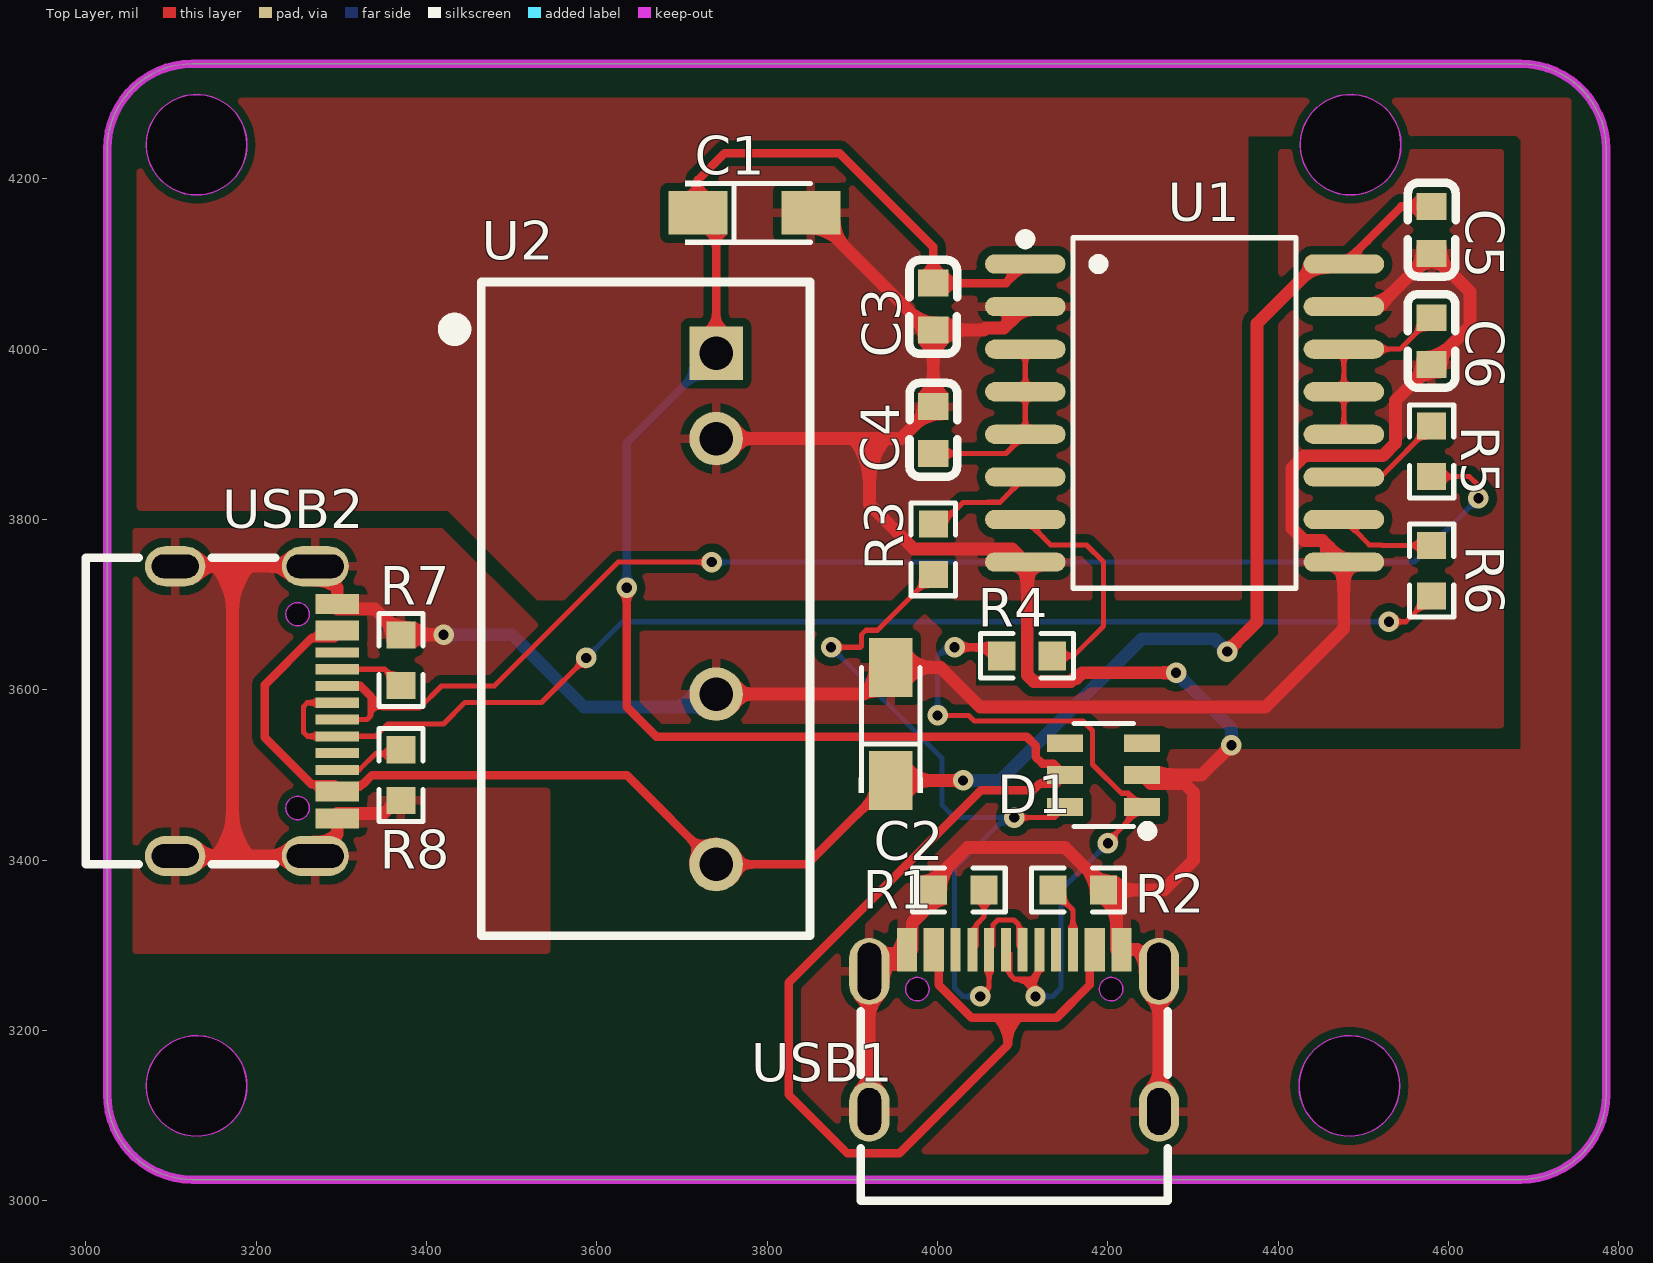
[diagram p0: Top Layer view]
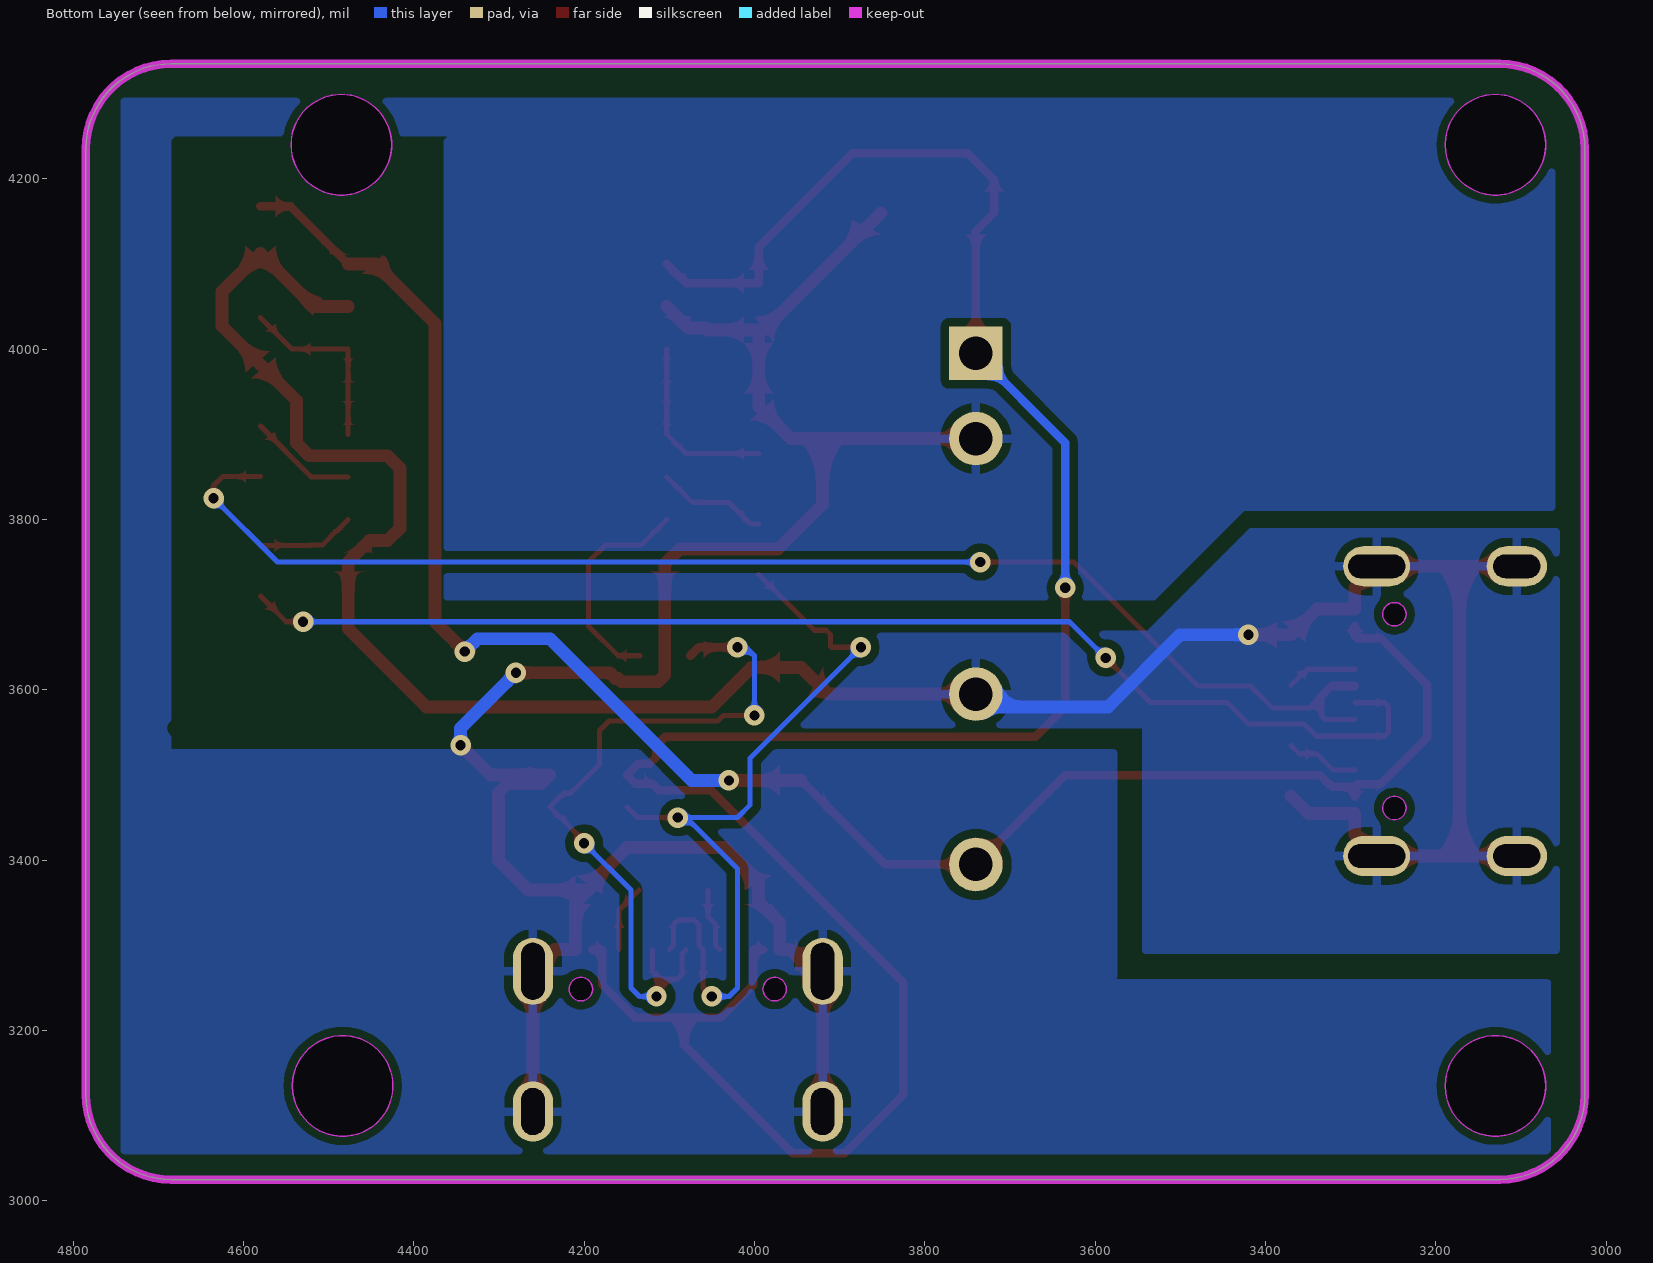
[diagram p1: Bottom Layer view, seen from below]
# Altium PCB MISC79005.pcbdoc
Units mil, origin at the board's own origin, x right, y up, seen from the top; angles counter-clockwise.
Board outline 1760 x 1310 mil, 2 copper layers (Top Layer, Bottom Layer), stack 62.206 mil thick; 19 components, 18 nets, 94 pads, 17 vias.

## Layer stack, top to bottom
Top Solder Mask Layer: solder mask 0.394, Dk 3.3
Top Layer: signal copper 1.379
Dielectric1: surface 59.449, FR4, Dk 4.5
Bottom Layer: signal copper 1.378
Bottom Solder Mask Layer: solder mask 0.394, Dk 3.3

## Board outline
3125,4335 ccw(c3125,4235) 3025,4235 3025,3125 ccw(c3125,3125) 3125,3025 4685,3025 ccw(c4685,3125) 4785,3125 4785,4235 ccw(c4685,4235) 4685,4335
cut-out: 3189.1,4240 cw(c3130,4240) 3070.9,4240 cw(c3130,4240)
cut-out: 4544.1,4240 cw(c4485,4240) 4425.9,4240 cw(c4485,4240)
cut-out: 3189.1,3135 cw(c3130,3135) 3070.9,3135 cw(c3130,3135)
cut-out: 4542.59,3135 cw(c4483.49,3135) 4424.39,3135 cw(c4483.49,3135)

## Design rules (kind name [scope] priority, off if disabled: settings)
BoardOutlineClearance copperThickness2oz_1 [All] p2 off: genericclearance=7.99 ignorepadtopadclearanceinfootprint=FALSE except(0: Arc-SplitContinuation Track-SplitContinuation SMDPad-SplitContinuation THPad-SplitContinuation Via-SplitContinuation Fill-SplitContinuation Region-SplitContinuation Poly-SplitContinuation Text-SplitContinuation Hole-SplitContinuation; 5.98: Arc-CutoutEdge Track-CutoutEdge SMDPad-CutoutEdge THPad-CutoutEdge Via-CutoutEdge Text-CutoutEdge; 6.9: Hole-OutlineEdge Hole-CutoutEdge; 10: Poly-OutlineEdge Poly-CutoutEdge; 11.81: Arc-OutlineEdge Track-OutlineEdge SMDPad-OutlineEdge THPad-OutlineEdge Via-OutlineEdge Fill-OutlineEdge Region-OutlineEdge Text-OutlineEdge Fill-CutoutEdge Region-CutoutEdge)
BoardOutlineClearance Plane_innerPlane_1 [All] p4 off: genericclearance=4.02 ignorepadtopadclearanceinfootprint=FALSE except(0: Arc-SplitContinuation Track-SplitContinuation SMDPad-SplitContinuation THPad-SplitContinuation Via-SplitContinuation Fill-SplitContinuation Region-SplitContinuation Poly-SplitContinuation Text-SplitContinuation Hole-SplitContinuation; 5.98: Arc-CutoutEdge Track-CutoutEdge SMDPad-CutoutEdge THPad-CutoutEdge Via-CutoutEdge Text-CutoutEdge; 6.9: Hole-OutlineEdge Hole-CutoutEdge; 10: Poly-OutlineEdge Poly-CutoutEdge; 11.81: Arc-OutlineEdge Track-OutlineEdge SMDPad-OutlineEdge THPad-OutlineEdge Via-OutlineEdge Fill-OutlineEdge Region-OutlineEdge Text-OutlineEdge Fill-CutoutEdge Region-CutoutEdge)
BoardOutlineClearance Copper_copperRegion_1 [All] p6 off: genericclearance=4.02 ignorepadtopadclearanceinfootprint=FALSE except(0: Arc-SplitContinuation Track-SplitContinuation SMDPad-SplitContinuation THPad-SplitContinuation Via-SplitContinuation Fill-SplitContinuation Region-SplitContinuation Poly-SplitContinuation Text-SplitContinuation Hole-SplitContinuation; 5.98: Arc-CutoutEdge Track-CutoutEdge SMDPad-CutoutEdge THPad-CutoutEdge Via-CutoutEdge Text-CutoutEdge; 6.9: Hole-OutlineEdge Hole-CutoutEdge; 10: Poly-OutlineEdge Poly-CutoutEdge; 11.81: Arc-OutlineEdge Track-OutlineEdge SMDPad-OutlineEdge THPad-OutlineEdge Via-OutlineEdge Fill-OutlineEdge Region-OutlineEdge Text-OutlineEdge Fill-CutoutEdge Region-CutoutEdge)
BoardOutlineClearance copperThickness1oz_1 [All] p8: genericclearance=4.02 ignorepadtopadclearanceinfootprint=FALSE except(0: Arc-SplitContinuation Track-SplitContinuation SMDPad-SplitContinuation THPad-SplitContinuation Via-SplitContinuation Fill-SplitContinuation Region-SplitContinuation Poly-SplitContinuation Text-SplitContinuation Hole-SplitContinuation; 5.98: Arc-CutoutEdge Track-CutoutEdge SMDPad-CutoutEdge THPad-CutoutEdge Via-CutoutEdge Text-CutoutEdge; 6.9: Hole-OutlineEdge Hole-CutoutEdge; 10: Poly-OutlineEdge Poly-CutoutEdge; 11.81: Arc-OutlineEdge Track-OutlineEdge SMDPad-OutlineEdge THPad-OutlineEdge Via-OutlineEdge Fill-OutlineEdge Region-OutlineEdge Text-OutlineEdge Fill-CutoutEdge Region-CutoutEdge)
Clearance copperThickness2oz [All] p1 off: gap=7.99 ignorepadtopadclearanceinfootprint=FALSE except(5.98: SMDPad-Track SMDPad-SMDPad THPad-Track SMDPad-THPad THPad-THPad Track-Via SMDPad-Via THPad-Via Via-Via Fill-SMDPad Region-SMDPad Fill-THPad Region-THPad Fill-Via Region-Via Fill-Fill Fill-Region Region-Region Arc-Track Arc-SMDPad Arc-THPad Arc-Via Fill-Arc Region-Arc Arc-Arc Text-Track SMDPad-Text Text-THPad Text-Via Fill-Text Region-Text Arc-Text Text-Text; 6.9: Hole-Track Hole-SMDPad Hole-THPad Hole-Via Fill-Hole Region-Hole Hole-Arc Hole-Text; 10: Poly-Track Poly-SMDPad Poly-THPad Poly-Via Poly-Fill Poly-Region Poly-Poly Poly-Arc Poly-Text Poly-Hole; 11.81: Fill-Track Region-Track)
Clearance Plane_innerPlane [All] p3 off: gap=4.02 ignorepadtopadclearanceinfootprint=FALSE except(5.98: SMDPad-Track SMDPad-SMDPad THPad-Track SMDPad-THPad THPad-THPad Track-Via SMDPad-Via THPad-Via Via-Via Fill-SMDPad Region-SMDPad Fill-THPad Region-THPad Fill-Via Region-Via Fill-Fill Fill-Region Region-Region Arc-Track Arc-SMDPad Arc-THPad Arc-Via Fill-Arc Region-Arc Arc-Arc Text-Track SMDPad-Text Text-THPad Text-Via Fill-Text Region-Text Arc-Text Text-Text; 6.9: Hole-Track Hole-SMDPad Hole-THPad Hole-Via Fill-Hole Region-Hole Hole-Arc Hole-Text; 10: Poly-Track Poly-SMDPad Poly-THPad Poly-Via Poly-Fill Poly-Region Poly-Poly Poly-Arc Poly-Text Poly-Hole; 11.81: Fill-Track Region-Track)
Clearance Copper_copperRegion [All] p5 off: gap=4.02 ignorepadtopadclearanceinfootprint=FALSE except(5.98: SMDPad-Track SMDPad-SMDPad THPad-Track SMDPad-THPad THPad-THPad Track-Via SMDPad-Via THPad-Via Via-Via Fill-SMDPad Region-SMDPad Fill-THPad Region-THPad Fill-Via Region-Via Fill-Fill Fill-Region Region-Region Arc-Track Arc-SMDPad Arc-THPad Arc-Via Fill-Arc Region-Arc Arc-Arc Text-Track SMDPad-Text Text-THPad Text-Via Fill-Text Region-Text Arc-Text Text-Text; 6.9: Hole-Track Hole-SMDPad Hole-THPad Hole-Via Fill-Hole Region-Hole Hole-Arc Hole-Text; 10: Poly-Track Poly-SMDPad Poly-THPad Poly-Via Poly-Fill Poly-Region Poly-Poly Poly-Arc Poly-Text Poly-Hole; 11.81: Fill-Track Region-Track)
Clearance copperThickness1oz [All] p7: gap=4.02 ignorepadtopadclearanceinfootprint=FALSE except(5.98: SMDPad-Track SMDPad-SMDPad THPad-Track SMDPad-THPad THPad-THPad Track-Via SMDPad-Via THPad-Via Via-Via Fill-SMDPad Region-SMDPad Fill-THPad Region-THPad Fill-Via Region-Via Fill-Fill Fill-Region Region-Region Arc-Track Arc-SMDPad Arc-THPad Arc-Via Fill-Arc Region-Arc Arc-Arc Text-Track SMDPad-Text Text-THPad Text-Via Fill-Text Region-Text Arc-Text Text-Text; 6.9: Hole-Track Hole-SMDPad Hole-THPad Hole-Via Fill-Hole Region-Hole Hole-Arc Hole-Text; 10: Poly-Track Poly-SMDPad Poly-THPad Poly-Via Poly-Fill Poly-Region Poly-Poly Poly-Arc Poly-Text Poly-Hole; 11.81: Fill-Track Region-Track)
DiffPairsRouting differentialPair [All] p1: maxlimit=6 minlimit=6 mostfreqgap=6 toplayer_minwidth=5 toplayer_prefwidth=10 toplayer_maxwidth=100 toplayer_mingap=6 toplayer_prefgap=6 toplayer_maxgap=6 bottomlayer_minwidth=5 bottomlayer_prefwidth=10 bottomlayer_maxwidth=100 bottomlayer_mingap=6 bottomlayer_prefgap=6 bottomlayer_maxgap=6 maxuncoupledlength=10
HoleToHoleClearance otherClearance [All] p1: gap=11.81 allowstackedmicrovias=TRUE
Length netLength [All] p1: minlimit=0 maxlimit=0
PasteMaskExpansion pasteMaskExpansion [All] p1: expansion=0
PlaneConnect innerPlane [All] p1: planeconnectstyle=Relief reliefexpansion=20 reliefentries=4 reliefconductorwidth=10 reliefairgap=10
PolygonConnect copperRegion [All] p1: connectstyle=Relief reliefconductorwidth=10 reliefentries=4 polygonreliefangle="90 Angle" airgapwidth=10 via.connectstyle=Relief via.reliefconductorwidth=10 via.reliefentries=4 via.polygonreliefangle="90 Angle" via.airgapwidth=10
RoutingVias viaSize [All] p1: holewidth=12.01 width=24.02 viastyle="Through Hole" minholewidth=11.81 minwidth=19.68 maxholewidth=248.03 maxwidth=393.7
SolderMaskExpansion solderMaskExpansion [IsVia] p1: expansion=-1000 istentingtop=TRUE
SolderMaskExpansion solderMaskExpansion [All] p2: expansion=2 istentingtop=FALSE
Width copperThickness2oz_2 [All] p1 off: maxlimit=100 minlimit=8 preferedwidth=10
Width copperThickness1oz_2 [All] p2: maxlimit=100 minlimit=5 preferedwidth=10

## Components (designator, comment, footprint, x,y, rotation, side; value= is the part's Value field where it differs from the comment)
C1 "10uF" CAP-SMD_L3.2-W1.6-RD-C7171 3785,4160 r0 top
C2 "10uF" CAP-SMD_L3.2-W1.6-RD-C7171 3945,3560 r90 top
C3 "100nF" C0603 3995,4050 r90 top
C4 "100nF" C0603 3995,3905 r270 top
C5 "100nF" C0603 4580,4140 r270 top
C6 "100nF" C0603 4579.79,4009.39 r270 top
D1 "SRV05-4HTG" SOT-23-6_L2.9-W1.6-P0.95-LS2.8-BL 4195,3500 r90 top
R1 "10K" R0603 4025,3365 r180 top
R2 "10K" R0603 4165,3365 r180 top
R3 "24Ω" R0603 3995,3765 r90 top
R4 "24Ω" R0603 4105,3640 r0 top
R5 "24Ω" R0603 4580,3880 r270 top
R6 "24Ω" R0603 4580,3740 r270 top
R7 "10K" R0603 3370,3635 r90 top
R8 "10K" R0603 3370,3500 r90 top
U1 "ADUM4160BRWZ-RL" SOIC-16_L10.3-W7.5-P1.27-LS10.3-BL 4290,3925 r270 top
U2 "H0505S-2WR2" PWRM-TH_EVISUN_HXXXXS-2WR2 3740,3695 r270 top
USB1 "KH-TYPE-C-16P" USB-C-SMD_KH-TYPE-C-16P#1 4090,3200 r0 top
USB2 "KH-TYPE-C-16P" USB-C-SMD_KH-TYPE-C-16P#2 3200,3575 r270 top

## Footprints (in the part's own frame and the unit in brackets; to place one, negate y for a bottom-side part, rotate by r counter-clockwise, add the part's x,y. Pads: shape width x height; smd on the part's side, far side on the other; paste and mask are expansions set on the pad)
C0603 [mm]
  rect 0.8x0.9 smd paste+0 mask+0.051: 1(-0.7,0) 2(0.7,0)
  silkscreen extent -1.41,-0.71 1.39,0.72
CAP-SMD_L3.2-W1.6-RD-C7171 [mil]
  rect 69.19x51.02 smd: 1(-66.39,0) 2(66.39,0)
  silkscreen extent -81,-37 66,37
PWRM-TH_EVISUN_HXXXXS-2WR2 [mm]
  rect 1.6x1.6 hole 1 paste+0 mask+0.05: 1(-7.62,0)
  round 1.6 hole 1 paste+0 mask+0.05: 2(-5.08,0) 5(2.54,0) 7(7.62,0)
  silkscreen extent -9.75,-8.05 9.75,2.8
R0603 [mil]
  rect 31.75x34.02 smd paste-3937.01 mask+2: 1(-29.66,0) 2(29.66,0)
  silkscreen extent -55,-26 55,26
SOIC-16_L10.3-W7.5-P1.27-LS10.3-BL [mil]
  oval 22.6x94.51 smd paste+0 mask+2: 1(-175,-187.02) 2(-125,-187.02) 3(-75,-187.02) 4(-25,-187.02) 5(25,-187.02) 6(75,-187.02) 7(125,-187.02) 8(175,-187.02) 9(175,187.02) 10(125,187.02) 11(75,187.02) 12(25,187.02) 13(-25,187.02) 14(-75,187.02) 15(-125,187.02) 16(-175,187.02)
  silkscreen extent -210,-193 206,131
SOT-23-6_L2.9-W1.6-P0.95-LS2.8-BL [mil]
  rect 20.95x42.2 smd: 1(-37.4,-45.24) 2(0,-45.24) 3(37.4,-45.24) 4(37.4,45.24) 5(0,45.24) 6(-37.4,45.24)
  silkscreen extent -72,-57 61,35
USB-C-SMD_KH-TYPE-C-16P#1 [mm]
  oval 1.2x2 hole 0.7 slot 1.7 at 90 deg: 1(-4.32,1.765) 2(4.32,1.765)
  oval 1.2x1.8 hole 0.7 slot 1.4 at 90 deg: 3(-4.32,-2.415) 4(4.32,-2.415)
  rect 0.3x1.3 smd paste-100 mask+0.05: A1(-3.35,2.415) A4(-2.55,2.415) A5(-1.25,2.415) A6(-0.25,2.415) A7(0.25,2.415) A8(1.25,2.415) A9(2.55,2.415) A12(3.35,2.415) B1(3.05,2.415) B4(2.25,2.415) B5(1.75,2.415) B6(0.75,2.415) B7(-0.75,2.415) B8(-1.75,2.415) B9(-2.25,2.415) B12(-3.05,2.415)
  Board Outline Layer circle w0.003: c-2.89,1.235 r0.35
  Board Outline Layer circle w0.003: c2.89,1.235 r0.35
  Board Outline Layer region: -2.54,1.235 -2.575,1.083 -2.672,0.961 -2.812,0.894 -2.968,0.894 -3.108,0.961 -3.205,1.083 -3.24,1.235 -3.24,1.235 -3.205,1.387 -3.108,1.509 -2.968,1.576 -2.812,1.576 -2.672,1.509 -2.575,1.387 -2.54,1.235
  Board Outline Layer region: -2.54,1.235 -2.549,1.157 -2.575,1.083 -2.616,1.017 -2.672,0.961 -2.738,0.92 -2.812,0.894 -2.89,0.885 -2.968,0.894 -3.042,0.92 -3.108,0.961 -3.164,1.017 -3.205,1.083 -3.231,1.157 -3.24,1.235 -3.231,1.313 -3.205,1.387 -3.164,1.453 -3.108,1.509 -3.042,1.55 -2.968,1.576 -2.89,1.585 -2.812,1.576 -2.738,1.55 -2.672,1.509 -2.616,1.453 -2.575,1.387 -2.549,1.313
  Board Outline Layer region: 3.24,1.235 3.205,1.083 3.108,0.961 2.968,0.894 2.812,0.894 2.672,0.961 2.575,1.083 2.54,1.235 2.54,1.235 2.575,1.387 2.672,1.509 2.812,1.576 2.968,1.576 3.108,1.509 3.205,1.387 3.24,1.235
  Board Outline Layer region: 3.24,1.235 3.231,1.157 3.205,1.083 3.164,1.017 3.108,0.961 3.042,0.92 2.968,0.894 2.89,0.885 2.812,0.894 2.738,0.92 2.672,0.961 2.616,1.017 2.575,1.083 2.549,1.157 2.54,1.235 2.549,1.313 2.575,1.387 2.616,1.453 2.672,1.509 2.738,1.55 2.812,1.576 2.89,1.585 2.968,1.576 3.042,1.55 3.108,1.509 3.164,1.453 3.205,1.387 3.231,1.313
  Multi-Layer board cut-out: -2.54,1.235 -2.575,1.083 -2.672,0.961 -2.812,0.894 -2.968,0.894 -3.108,0.961 -3.205,1.083 -3.24,1.235 -3.24,1.235 -3.205,1.387 -3.108,1.509 -2.968,1.576 -2.812,1.576 -2.672,1.509 -2.575,1.387 -2.54,1.235
  Multi-Layer board cut-out: 3.24,1.235 3.205,1.083 3.108,0.961 2.968,0.894 2.812,0.894 2.672,0.961 2.575,1.083 2.54,1.235 2.54,1.235 2.575,1.387 2.672,1.509 2.812,1.576 2.968,1.576 3.108,1.509 3.205,1.387 3.24,1.235
  silkscreen extent -4.57,-5.08 4.57,0.57
USB-C-SMD_KH-TYPE-C-16P#2 [mm]
  oval 1.2x2 hole 0.7 slot 1.7 at 90 deg: 1(-4.32,1.765) 2(4.32,1.765)
  oval 1.2x1.8 hole 0.7 slot 1.4 at 90 deg: 3(-4.32,-2.415) 4(4.32,-2.415)
  rect 0.3x1.3 smd paste-100 mask+0.05: A1(-3.35,2.415) A4(-2.55,2.415) A5(-1.25,2.415) A6(-0.25,2.415) A7(0.25,2.415) A8(1.25,2.415) A9(2.55,2.415) A12(3.35,2.415) B1(3.05,2.415) B4(2.25,2.415) B5(1.75,2.415) B6(0.75,2.415) B7(-0.75,2.415) B8(-1.75,2.415) B9(-2.25,2.415) B12(-3.05,2.415)
  Board Outline Layer circle w0.003: c-2.89,1.235 r0.35
  Board Outline Layer circle w0.003: c2.89,1.235 r0.35
  Board Outline Layer region: -2.89,1.585 -2.738,1.55 -2.616,1.453 -2.549,1.313 -2.549,1.157 -2.616,1.017 -2.738,0.92 -2.89,0.885 -2.89,0.885 -3.042,0.92 -3.164,1.017 -3.231,1.157 -3.231,1.313 -3.164,1.453 -3.042,1.55 -2.89,1.585
  Board Outline Layer region: -2.89,1.585 -2.812,1.576 -2.738,1.55 -2.672,1.509 -2.616,1.453 -2.575,1.387 -2.549,1.313 -2.54,1.235 -2.549,1.157 -2.575,1.083 -2.616,1.017 -2.672,0.961 -2.738,0.92 -2.812,0.894 -2.89,0.885 -2.968,0.894 -3.042,0.92 -3.108,0.961 -3.164,1.017 -3.205,1.083 -3.231,1.157 -3.24,1.235 -3.231,1.313 -3.205,1.387 -3.164,1.453 -3.108,1.509 -3.042,1.55 -2.968,1.576
  Board Outline Layer region: 2.89,1.585 3.042,1.55 3.164,1.453 3.231,1.313 3.231,1.157 3.164,1.017 3.042,0.92 2.89,0.885 2.89,0.885 2.738,0.92 2.616,1.017 2.549,1.157 2.549,1.313 2.616,1.453 2.738,1.55 2.89,1.585
  Board Outline Layer region: 2.89,1.585 2.968,1.576 3.042,1.55 3.108,1.509 3.164,1.453 3.205,1.387 3.231,1.313 3.24,1.235 3.231,1.157 3.205,1.083 3.164,1.017 3.108,0.961 3.042,0.92 2.968,0.894 2.89,0.885 2.812,0.894 2.738,0.92 2.672,0.961 2.616,1.017 2.575,1.083 2.549,1.157 2.54,1.235 2.549,1.313 2.575,1.387 2.616,1.453 2.672,1.509 2.738,1.55 2.812,1.576
  Multi-Layer board cut-out: -2.89,1.585 -2.738,1.55 -2.616,1.453 -2.549,1.313 -2.549,1.157 -2.616,1.017 -2.738,0.92 -2.89,0.885 -2.89,0.885 -3.042,0.92 -3.164,1.017 -3.231,1.157 -3.231,1.313 -3.164,1.453 -3.042,1.55 -2.89,1.585
  Multi-Layer board cut-out: 2.89,1.585 3.042,1.55 3.164,1.453 3.231,1.313 3.231,1.157 3.164,1.017 3.042,0.92 2.89,0.885 2.89,0.885 2.738,0.92 2.616,1.017 2.549,1.157 2.549,1.313 2.616,1.453 2.738,1.55 2.89,1.585
  silkscreen extent -4.57,-5.08 4.57,0.57

## Via types
v1: diameter 24.02, hole 12, Top Layer to Bottom Layer, 17 vias

## Nets (pads, with @x,y where several pads share a name; then routed paths per layer and width w, separated by ;. In a path a pad name is that pad's centre, name@x,y a point inside that pad or via, vN(x,y) a via of type N, cw(c..) or ccw(c..) an arc to the next point about the centre after c; other vN are vias at no path point)
$1N543: R2.2 USB1.B5 | length 79.7
  Top Layer w6: R2.2 4158.9,3341.44 USB1.B5
$1N556: R1.1 USB1.A5 | length 75.7
  Top Layer w6: USB1.A5 4045.58,3299.87 4045.58,3324.4 4054.66,3333.48 R1.1
$1N991: C6.1 U1.12 U1.13 U1.14 | length 218.1
  Top Layer w6: U1.12 U1.13 U1.14 4542.84,4000 C6.1
$1N997: R5.1 U1.11 | length 127.7
  Top Layer w6: U1.11 4520.34,3850 R5.1
$1N998: R6.1 U1.10 | length 115.5
  Top Layer w6: U1.10 4506.74,3770.29 4521.38,3770.29 4522,3769.66 R6.1
$1N1000: C4.2 U1.3 U1.4 U1.5 | length 217.3
  Top Layer w6: C4.2 4080.42,3877.44 U1.5 U1.4 U1.3
$1N1002: R3.2 U1.6 | length 130.9
  Top Layer w6: R3.2 4004.66,3794.66 4030,3820 4058.34,3820 4058.63,3820.29 4073.27,3820.29 U1.6
$1N1003: R4.2 U1.7 | length 262.6
  Top Layer w6: U1.7 4132.7,3770.29 4147.34,3770.29 4147.62,3770 4175,3770 4195,3750 4195,3675 4160,3640 R4.2
$1N2241: R8.2 USB2.B5 | length 86.7
  Top Layer w6: USB2.B5 3321.1,3506.1 3340,3525 3360.34,3525 R8.2@3370,3534.66
$1N2257: R7.1 USB2.A5 | length 82.7
  Top Layer w6: USB2.A5 3351.13,3624.21 R7.1
+5V: C2.1 C5.1 U1.16 U2.7 USB2.A4 USB2.A9 USB2.B4 USB2.B9 | length 2174.8
  Top Layer w10: USB2.A9 USB2.B4 ; USB2.A4 USB2.B9 3292.29,3660.79 3264.94,3660.79 3210,3605.85 3210,3544.15 3264.94,3489.21 3292.28,3489.21 USB2.B4 ; C2.1 3846.39,3395 U2.7 3635,3500 3336.01,3500 3325.22,3489.21 3324.21,3489.21 3321.42,3486.42 USB2.B4 ; U1.16 4544.58,4167.56 C5.1
  Top Layer w15: C2.1 v1(4030,3493.61) ; v1(4340,3645) 4375,3680 4375,4030 4445,4100 U1.16
  Bottom Layer w15: v1(4030,3493.61) 4073.61,3493.61 4240,3660 4325,3660 v1(4340,3645)
+5V-USB: C1.1 C3.2 D1.5 U1.1 U2.1 USB1.A4 USB1.A9 USB1.B4 USB1.B9 | length 2964.7
  Top Layer w10: v1(3635,3720) 3635,3580 3670,3545 4104.76,3545 4115.18,3534.59 4115.18,3521.35 4123.08,3513.45 4136.32,3513.45 D1.5 4139.76,3490 4120,3490 4112.06,3482.06 4050.97,3482.06 3825,3256.1 3825,3125 3894.25,3055.76 3955,3055.76 4082.64,3183.4 4082.64,3215 ; U2.1 3740,4138.61 C1.1 3718.61,4198.61 3750,4230 3885,4230 3995,4120 C3.2 4080.54,4077.56 U1.1 ; USB1.A4 USB1.B9 4001.42,3253.58 4040,3215 4082.64,3215 ; USB1.A9 USB1.B4 4178.58,3253.58 4140,3215 4082.64,3215
  Bottom Layer w10: v1(3635,3720) 3635,3890 U2.1
D+: R6.2 USB2.A6 USB2.B6 | length 1466.1
  Top Layer w6: USB2.A6 3260,3584.84 3255.76,3580.6 3255.76,3550 3260.29,3545.47 USB2.B6 3340.22,3545.47 3354.75,3560 3420,3560 3445,3585 3535,3585 v1(3587.5,3637.5) ; v1(4530,3680) 4549.66,3680 R6.2
  Bottom Layer w6: v1(3587.5,3637.5) 3630,3680 v1(4530,3680)
D-: R5.2 USB2.A7 USB2.B7 | length 1591.3
  Top Layer w6: USB2.A7 3330,3565.16 3334.25,3569.41 3334.25,3592.68 3348.45,3578.48 3391.56,3578.48 3417.61,3604.53 3479.53,3604.53 3625,3750 v1(3735,3750) ; R5.2 4624.66,3850.34 4635,3840 v1(4635,3825)
  Top Layer w10: USB2.B7 3322.4,3604.53 3334.25,3592.68
  Bottom Layer w6: v1(3735,3750) 4560,3750 v1(4635,3825)
GND: C2.2 C5.2 C6.2 R7.2 R8.1 U1.9 U1.15 U2.5 USB2.1 USB2.2 USB2.3 USB2.4 USB2.A1 USB2.A12 USB2.B1 USB2.B12 | length 2946.8
  Top Layer w15: USB2.4 3174.67,3404.92 ; USB2.3 3172.19,3745.08 ; R8.1@3370,3475.34 3349.58,3454.92 USB2.B1 USB2.A12 3295.08,3430.51 USB2.2 3174.67,3404.92 ; v1(3420,3664.66) R7.2 3339.58,3695.08 USB2.B12 USB2.A1 3295.08,3719.49 USB2.1 3172.19,3745.08 ; U2.5 3913.61,3595 C2.2 4003.61,3626.39 4050,3580 4385,3580 4477.02,3672.02 U1.9 4451.81,3775.22 4430.8,3775.22 4416.29,3789.74 4416.29,3860.27 4430.8,3874.79 4522.81,3874.79 4537.76,3889.74 4537.76,3939.81 C6.2 4625,4027.05 4625,4067.44 C5.2 4517.56,4050 U1.15 ; 3172.19,3745.08 3172.19,3407.4 3174.67,3404.92
  Bottom Layer w15: v1(3420,3664.66) 3500.34,3664.66 3585,3580 3725,3580 U2.5
GND-USB: C1.2 C3.1 C4.1 D1.2 R1.2 R2.1 U1.2 U1.8 U2.2 USB1.1 USB1.2 USB1.3 USB1.4 USB1.A1 USB1.A12 USB1.B1 USB1.B12 | length 2637.5
  Top Layer w15: U2.2 3917.35,3895 ; C1.2 3988.95,4022.44 C3.1 ; USB1.3 USB1.1 3932.52,3269.49 USB1.A1 USB1.B12 3970.22,3295.38 3970.22,3326.26 3995.34,3351.38 R1.2@3995.34,3360 ; R1.2 3995.34,3375.34 4035,3415 4149.66,3415 4189.66,3375 4189.66,3370 R2.1 ; U1.2 4077.77,4024.79 4056.76,4024.79 4054.42,4022.44 C3.1 ; USB1.4 USB1.2 4234.49,3295.08 USB1.A12 USB1.B1 4210.08,3349.58 R2.1 ; v1(4280,3620) 4169.85,3620 4163.04,3613.19 4159.81,3613.19 4156.12,3609.51 4113.2,3609.51 4105.3,3617.41 4105.3,3747.68 U1.8 4087.68,3765.3 3972.41,3765.3 3920,3817.71 3920,3892.35 3917.35,3895 ; v1(4345,3535) 4310,3500 D1.2 4250.24,3490 4290,3490 4300.61,3479.4 4300.61,3400 4265.61,3365 R2.1 ; 3917.35,3895 3957.44,3895 C4.1 C3.1
  Bottom Layer w15: v1(4280,3620) 4345,3555 v1(4345,3535)
UD+: D1.1 R4.1 USB1.A6 USB1.B6 | length 870
  Top Layer w6: v1(4000,3570) 4036.65,3570 4043.16,3563.49 4170.79,3563.49 4181.85,3552.43 4181.85,3512.51 4215.82,3478.55 4224.3,3478.55 D1.1 4200,3422.36 v1(4200,3420) ; USB1.A6 4084.95,3290.29 4084.95,3265.77 4090.72,3260 4110,3260 4111.98,3261.98 ; 4111.98,3263.02 4111.98,3261.98 ; v1(4115,3240) 4111.98,3243.02 4111.98,3261.98 ; USB1.B6 4119.53,3269.53 4111.98,3261.98
  Top Layer w10: v1(4020,3650) 4065.34,3650 R4.1
  Bottom Layer w6: v1(4000,3570) 4000,3640 4010,3650 v1(4020,3650) ; v1(4115,3240) 4135,3240 4145,3250 4145,3365 v1(4200,3420)
UD-: D1.6 R3.1 USB1.A7 USB1.B7 | length 973.7
  Top Layer w6: v1(3875,3650) 3909.66,3650 3910.51,3650.85 3910.51,3664.71 3915.77,3669.97 3929.63,3669.97 R3.1 ; v1(4050,3240) 4060.47,3250.47 USB1.B7 4065.27,3299.88 4065.27,3324.4 4070.54,3329.66 4089.79,3329.66 4095.05,3324.4 4095.05,3299.87 USB1.A7 ; v1(4090,3450) 4137.16,3450 D1.6
  Bottom Layer w6: v1(3875,3650) 4005,3520 4005,3465 4020,3450 v1@4080,3450 ; v1(4050,3240) 4030,3240 4020,3250 4020,3390 v1@4080,3450 ; v1(4090,3450) v1@4080,3450
pads on no net: D1.3 D1.4 USB1.A8 USB1.B8 USB2.A8 USB2.B8

## Polygon pours and split planes (outlines as drawn)
GND on Top Layer (solid, remove dead copper, pour order 0): 3055,3790 3418.67,3790 3539.34,3669.34 3964.34,3669.34 3985,3690 4045,3630 4045,3605 4340,3605 4400,3665 4400,4235 4665,4235 4665,3555 3545,3555 3545,3290 3055,3290
GND on Bottom Layer (solid, remove dead copper, pour order 4): 3054.7,3790 3418.37,3790 3539.04,3669.34 3964.04,3669.34 3984.7,3690 4044.7,3630 4044.7,3605 4339.7,3605 4399.7,3665 4399.7,4235 4624.7,4235 4664.7,4195 4664.7,3570 4679.7,3555 3544.7,3555 3544.7,3290 3054.7,3290
GND-USB on Top Layer (solid, remove dead copper, pour order 2): 3060,3810 3425,3810 3530,3705 4365,3705 4365,4250 4680,4250 4685,4245 4685,3530 3574.14,3530 3574.14,3260.87 3575,3260 3070,3260 3065,3265 3065,3060 3060,3055 4744.29,3055 4744.29,4295 3060,4295
GND-USB on Bottom Layer (solid, remove dead copper, pour order 6): 3060,3810 3425,3810 3530,3705 4365,3705 4365,4245 4360,4250 4680,4250 4685,4245 4685,3530 3574.14,3530 3574.14,3260.87 3575,3260 3070,3260 3065,3265 3065,3060 3060,3055 4744.29,3055 4744.29,4295 3060,4295

## Keep-outs
Board Outline Layer:
  region: 3189.1,4240 cw(c3130,4240) 3070.9,4240 cw(c3130,4240)
  circle w0.1: c3130,4240 r59.1
  region: 3189.1,4240 3188.7,4233.14 3187.51,4226.37 3185.54,4219.79 3182.82,4213.48 3179.38,4207.53 3175.28,4202.02 3170.56,4197.02 3165.3,4192.6 3159.55,4188.82 3153.41,4185.74 3146.95,4183.39 3140.27,4181.8 3133.44,4181 3126.57,4181 3119.74,4181.8 3113.05,4183.39 3106.6,4185.74 3100.45,4188.82 3094.71,4192.6 3089.45,4197.02 3084.73,4202.02 3080.63,4207.53 3077.19,4213.48 3074.47,4219.79 3072.5,4226.37 3071.3,4233.14 3070.9,4240 3071.3,4246.87 3072.5,4253.63 3074.47,4260.22 3077.19,4266.53 3080.63,4272.48 3084.73,4277.99 3089.45,4282.99 3094.71,4287.41 3100.45,4291.19 3106.6,4294.27 3113.05,4296.62 3119.74,4298.21 3126.57,4299 3133.44,4299 3140.27,4298.21 3146.95,4296.62 3153.41,4294.27 3159.55,4291.19 3165.3,4287.41 3170.56,4282.99 3175.28,4277.99 3179.38,4272.48 3182.82,4266.53 3185.54,4260.22 3187.51,4253.63 3188.7,4246.87
  region: 4544.1,4240 cw(c4485,4240) 4425.9,4240 cw(c4485,4240)
  circle w0.1: c4485,4240 r59.1
  region: 4544.1,4240 4543.7,4233.14 4542.51,4226.37 4540.54,4219.79 4537.82,4213.48 4534.38,4207.53 4530.28,4202.02 4525.56,4197.02 4520.3,4192.6 4514.55,4188.82 4508.41,4185.74 4501.95,4183.39 4495.27,4181.8 4488.44,4181 4481.57,4181 4474.74,4181.8 4468.05,4183.39 4461.6,4185.74 4455.45,4188.82 4449.71,4192.6 4444.45,4197.02 4439.73,4202.02 4435.63,4207.53 4432.19,4213.48 4429.47,4219.79 4427.5,4226.37 4426.3,4233.14 4425.9,4240 4426.3,4246.87 4427.5,4253.63 4429.47,4260.22 4432.19,4266.53 4435.63,4272.48 4439.73,4277.99 4444.45,4282.99 4449.71,4287.41 4455.45,4291.19 4461.6,4294.27 4468.05,4296.62 4474.74,4298.21 4481.57,4299 4488.44,4299 4495.27,4298.21 4501.95,4296.62 4508.41,4294.27 4514.55,4291.19 4520.3,4287.41 4525.56,4282.99 4530.28,4277.99 4534.38,4272.48 4537.82,4266.53 4540.54,4260.22 4542.51,4253.63 4543.7,4246.87
  region: 3189.1,3135 cw(c3130,3135) 3070.9,3135 cw(c3130,3135)
  circle w0.1: c3130,3135 r59.1
  region: 3189.1,3135 3188.7,3128.14 3187.51,3121.37 3185.54,3114.79 3182.82,3108.48 3179.38,3102.53 3175.28,3097.02 3170.56,3092.02 3165.3,3087.6 3159.55,3083.82 3153.41,3080.74 3146.95,3078.39 3140.27,3076.8 3133.44,3076 3126.57,3076 3119.74,3076.8 3113.05,3078.39 3106.6,3080.74 3100.45,3083.82 3094.71,3087.6 3089.45,3092.02 3084.73,3097.02 3080.63,3102.53 3077.19,3108.48 3074.47,3114.79 3072.5,3121.37 3071.3,3128.14 3070.9,3135 3071.3,3141.87 3072.5,3148.63 3074.47,3155.22 3077.19,3161.53 3080.63,3167.48 3084.73,3172.99 3089.45,3177.99 3094.71,3182.41 3100.45,3186.19 3106.6,3189.27 3113.05,3191.62 3119.74,3193.21 3126.57,3194 3133.44,3194 3140.27,3193.21 3146.95,3191.62 3153.41,3189.27 3159.55,3186.19 3165.3,3182.41 3170.56,3177.99 3175.28,3172.99 3179.38,3167.48 3182.82,3161.53 3185.54,3155.22 3187.51,3148.63 3188.7,3141.87
  region: 4542.59,3135 cw(c4483.49,3135) 4424.39,3135 cw(c4483.49,3135)
  circle w0.1: c4483.49,3135 r59.1
  region: 4542.59,3135 4542.19,3128.14 4540.99,3121.37 4539.02,3114.79 4536.3,3108.48 4532.86,3102.53 4528.76,3097.02 4524.04,3092.02 4518.78,3087.6 4513.04,3083.82 4506.9,3080.74 4500.44,3078.39 4493.75,3076.8 4486.92,3076 4480.05,3076 4473.22,3076.8 4466.54,3078.39 4460.08,3080.74 4453.94,3083.82 4448.2,3087.6 4442.93,3092.02 4438.21,3097.02 4434.11,3102.53 4430.67,3108.48 4427.95,3114.79 4425.98,3121.37 4424.79,3128.14 4424.39,3135 4424.79,3141.87 4425.98,3148.63 4427.95,3155.22 4430.67,3161.53 4434.11,3167.48 4438.21,3172.99 4442.93,3177.99 4448.2,3182.41 4453.94,3186.19 4460.08,3189.27 4466.54,3191.62 4473.22,3193.21 4480.05,3194 4486.92,3194 4493.75,3193.21 4500.44,3191.62 4506.9,3189.27 4513.04,3186.19 4518.78,3182.41 4524.04,3177.99 4528.76,3172.99 4532.86,3167.48 4536.3,3161.53 4539.02,3155.22 4540.99,3148.63 4542.19,3141.87
  lines w10: 3025,3125 3025,4235 cw(c3125,4235) 3125,4335 4685,4335 cw(c4685,4235) 4785,4235 4785,3125 cw(c4685,3125) 4685,3025 3125,3025 cw(c3125,3125) 3025,3125

## Other copper
Top Layer:
  drawing of 126 lines, arcs and shapes, not listed
Bottom Layer:
  region net GND: 3710.89,3572.5 3688.39,3587.5 3690.21,3587.61 3692,3587.92 3693.76,3588.41 3695.48,3589.08 3697.15,3589.91 3698.77,3590.89 3701.81,3593.24 3704.56,3596.02 3706.94,3599.12 3708.92,3602.43 3710.44,3605.85 3732.94,3564.31 3729.81,3565.25 3727.02,3566.46 3722,3569.18 3719.53,3570.45 3716.93,3571.51 3714.09,3572.24
  region net +5V-USB: 3710.28,3958.2 3703.2,3965.28 3705.48,3968.88 3707.15,3972.8 3708.17,3976.94 3708.51,3981.19 3726.19,3963.51 3721.94,3963.17 3717.8,3962.15 3713.88,3960.48 3710.28,3958.2
  region net +5V-USB: 3630,3736.35 3640,3736.35 3640.09,3735.21 3640.35,3734.08 3641.26,3731.87 3642.54,3729.79 3644.01,3727.95 3626,3727.95 3627.47,3729.79 3628.75,3731.87 3629.66,3734.08 3629.91,3735.21
  region net D-: 3751.35,3753 3751.35,3747 3749.83,3746.87 3748.6,3746.49 3747.6,3745.9 3746.72,3745.13 3745.06,3743.2 3742.95,3741 3742.95,3759.01 3745.06,3756.8 3746.72,3754.88 3747.6,3754.11 3748.6,3753.52 3749.83,3753.14
  region net D-: 4625.57,3811.32 4621.32,3815.57 4622.31,3816.74 4622.9,3817.87 4623.2,3819.01 4623.27,3820.17 4623.09,3822.7 4623.02,3825.76 4635.76,3813.02 4632.7,3813.09 4630.17,3813.27 4629.01,3813.2 4627.87,3812.9 4626.74,3812.31
  region net D+: 3596.94,3651.19 3601.19,3646.94 3600.2,3645.77 3599.61,3644.63 3599.31,3643.5 3599.24,3642.34 3599.42,3639.8 3599.49,3636.75 3586.75,3649.49 3589.8,3649.42 3592.34,3649.24 3593.5,3649.31 3594.63,3649.61 3595.77,3650.2
  region net D+: 4513.66,3677 4513.66,3683 4515.18,3683.14 4516.41,3683.52 4517.41,3684.11 4518.28,3684.88 4519.95,3686.8 4522.06,3689.01 4522.06,3671 4519.95,3673.2 4518.28,3675.13 4517.41,3675.9 4516.41,3676.49 4515.18,3676.87
  region net +5V: 4046.35,3501.11 4046.35,3486.11 4043.98,3486.19 4041.84,3486.19 4040.83,3486.06 4039.85,3485.78 4038.89,3485.31 4037.95,3484.61 4037.95,3502.62 4038.89,3501.92 4039.85,3501.45 4040.83,3501.17 4041.84,3501.04 4043.98,3501.04
  region net +5V: 4323.14,3651.26 4333.75,3661.87 4335.37,3660.14 4336.89,3658.62 4337.69,3658 4338.58,3657.51 4339.59,3657.16 4340.76,3656.99 4328.02,3644.25 4327.85,3645.42 4327.5,3646.42 4327.01,3647.31 4326.39,3648.12 4324.87,3649.64
  region net UD-: 4072.82,3438.58 4076.15,3450.39 4077.11,3451.44 4077.77,3452.35 4078.57,3453.93 4079.31,3455.56 4080.76,3457.67 4083.15,3440.14 4081.95,3440.78 4080.64,3441.14 4079.25,3441.24 4077.83,3441.11 4076.44,3440.76 4075.1,3440.21 4073.89,3439.47
  region net UD-: 4073.66,3447 4073.66,3453 4075.18,3453.14 4076.41,3453.52 4077.41,3454.11 4078.28,3454.88 4079.95,3456.8 4082.06,3459.01 4082.06,3441 4079.95,3443.2 4078.28,3445.13 4077.41,3445.9 4076.41,3446.49 4075.18,3446.87
  region net UD-: 4033.66,3237 4033.66,3243 4035.18,3243.14 4036.41,3243.52 4037.41,3244.11 4038.28,3244.88 4039.95,3246.8 4042.06,3249.01 4042.06,3231 4039.95,3233.2 4038.28,3235.13 4037.41,3235.9 4036.41,3236.49 4035.18,3236.87
  region net UD+: 4190.57,3406.32 4186.32,3410.57 4187.31,3411.74 4187.9,3412.87 4188.2,3414.01 4188.27,3415.17 4188.09,3417.7 4188.02,3420.76 4200.76,3408.02 4197.7,3408.09 4195.17,3408.27 4194.01,3408.2 4192.87,3407.9 4191.74,3407.31
  region net UD+: 4131.35,3243 4131.35,3237 4129.83,3236.87 4128.6,3236.49 4127.6,3235.9 4126.72,3235.13 4125.06,3233.2 4122.95,3231 4122.95,3249.01 4125.06,3246.8 4126.72,3244.88 4127.6,3244.11 4128.6,3243.52 4129.83,3243.14
  region net UD-: 3888.69,3640.57 3884.44,3636.32 3883.27,3637.31 3882.13,3637.9 3881,3638.2 3879.84,3638.27 3877.3,3638.09 3874.25,3638.02 3886.99,3650.76 3886.92,3647.7 3886.74,3645.17 3886.81,3644.01 3887.11,3642.87 3887.7,3641.74
  region net UD+: 3997,3586.35 4003,3586.35 4003.14,3584.83 4003.52,3583.6 4004.11,3582.6 4004.88,3581.72 4006.8,3580.06 4009.01,3577.95 3991,3577.95 3993.2,3580.06 3995.13,3581.72 3995.9,3582.6 3996.49,3583.6 3996.87,3584.83
  region net UD+: 4002.82,3638.58 4006.15,3650.39 4007.11,3651.44 4007.77,3652.35 4008.57,3653.93 4009.31,3655.56 4010.76,3657.67 4013.15,3640.14 4011.95,3640.78 4010.64,3641.14 4009.25,3641.24 4007.83,3641.11 4006.44,3640.76 4005.1,3640.21 4003.89,3639.47
  region net GND: 3436.35,3672.16 3436.35,3657.16 3433.98,3657.24 3431.84,3657.24 3430.83,3657.11 3429.85,3656.83 3428.89,3656.36 3427.95,3655.66 3427.95,3673.67 3428.89,3672.97 3429.85,3672.5 3430.83,3672.22 3431.84,3672.09 3433.98,3672.09
  region net GND-USB: 4337.5,3551.35 4352.5,3551.35 4352.43,3548.98 4352.43,3546.84 4352.56,3545.83 4352.84,3544.85 4353.31,3543.89 4354.01,3542.95 4336,3542.95 4336.7,3543.89 4337.17,3544.85 4337.45,3545.83 4337.58,3546.84 4337.58,3548.98
  region net GND-USB: 4296.87,3613.75 4286.26,3603.14 4284.64,3604.87 4283.12,3606.39 4282.31,3607.01 4281.42,3607.5 4280.42,3607.85 4279.25,3608.02 4291.99,3620.76 4292.16,3619.59 4292.51,3618.58 4293,3617.69 4293.62,3616.89 4295.14,3615.37

## Silkscreen, mask and mechanical layers (free items; w line width, h text height)
Mechanical Layer:
  circle w0.1: c3130,4240 r59.1
  circle w0.1: c4485,4240 r59.1
  circle w0.1: c3130,3135 r59.1
  circle w0.1: c4483.49,3135 r59.1